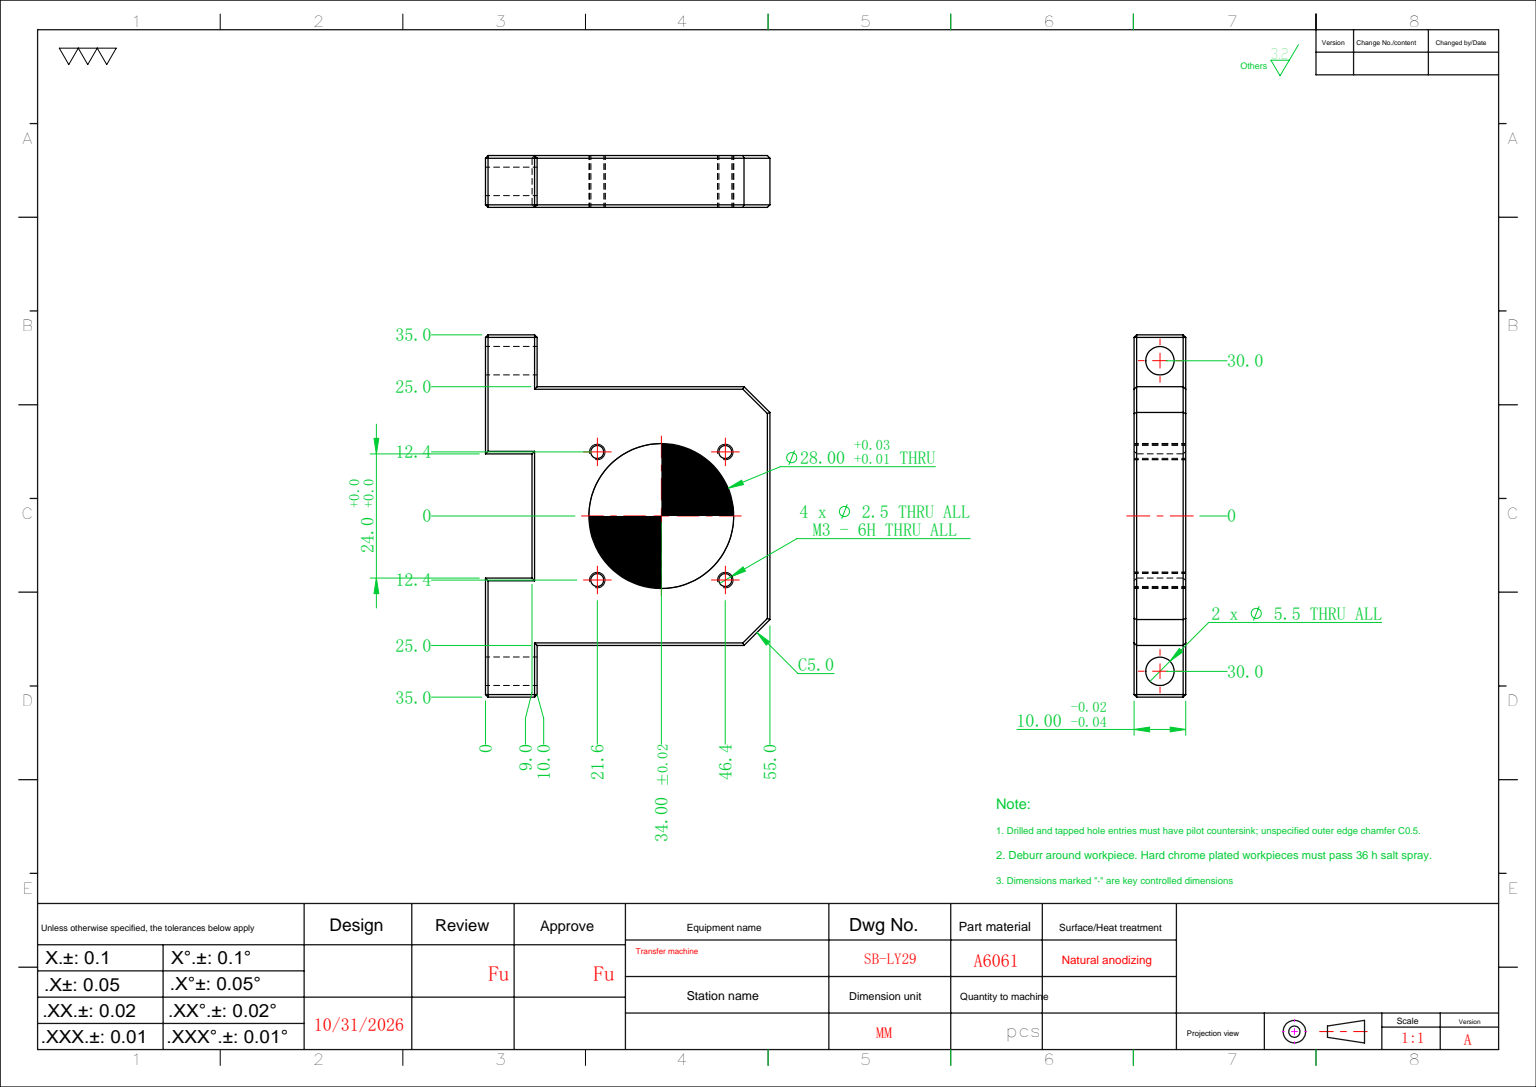
SolidWorks part; units mm, degrees
ref_plane "前视基准面" through (0, 0, 0) normal (0, 0, 1) x (1, 0, 0)
ref_plane "上视基准面" through (0, 0, 0) normal (0, 1, 0) x (1, 0, 0)
ref_plane "右视基准面" through (0, 0, 0) normal (1, 0, 0) x (0, 0, -1)
sketch "草图1" plane through (0, 0, 0) normal (0, 0, 1) x (1, 0, 0)
  line L1 (-35, -27.5) -> (35, -27.5)
  line L2 (-35, -27.5) -> (-35, 27.5)
  line L3 (-35, 27.5) -> (35, 27.5)
  line L4 (35, -27.5) -> (35, 27.5)
  line L5 (-35, -27.5) -> (35, 27.5) construction
  line L6 (-35, 27.5) -> (35, -27.5) construction
  point P0 (0, 0)
  dimension "D1" = 70
  dimension "D2" = 55
extrude "凸台-拉伸1" add sketch "草图1" along normal blind 10
sketch "草图2" plane through (0, 0, 10) normal (0, 0, 1) x (1, 0, 0)
  line L0 (0, 0) -> (0, -35.8295) construction
  line L1 (-35, -27.5) -> (-25, -27.5)
  line L2 (-35, -27.5) -> (-35, 17.5)
  line L3 (-35, 17.5) -> (-25, 17.5)
  line L4 (-25, -27.5) -> (-25, 17.5)
  line L5 (25, -27.5) -> (25, 17.5)
  line L6 (35, 17.5) -> (25, 17.5)
  line L7 (35, -27.5) -> (35, 17.5)
  line L8 (35, -27.5) -> (25, -27.5)
  line L9 (35, 27.5) -> (-35, 27.5) construction
  dimension "D1" = 10
  dimension "D2" = 10
extrude "切除-拉伸1" cut sketch "草图2" against normal through all
sketch "草图3" plane through (0, 0, 0) normal (0, 0, -1) x (-1, 0, 0)
  line L0 (0, 0) -> (0, -40.7468) construction
  line L1 (-35, 27.5) -> (35, 27.5) construction
  circle A0 centre (0, -6.5) radius 14
  dimension "D1" = 28
  dimension "D2" = 34
extrude "切除-拉伸2" cut sketch "草图3" against normal through all
hole_wizard "M3 螺纹孔1" positions "草图8" profile "草图9" tap size "M3" standard "ISO" end condition through all
sketch "草图8" plane through (0, 0, 10) normal (0, 0, 1) x (1, 0, 0)
  line L0 (0, -6.5) -> (0, -34.3856) construction
  line L3 (0, -6.5) -> (-29.4307, -6.5) construction
  point P0 (12.375, -18.875)
  point P2 (-12.375, -18.875)
  point P4 (-12.375, 5.875)
  point P6 (12.375, 5.875)
  dimension "D1" = 24.75
  dimension "D2" = 24.75
sketch "草图9" plane through (12.375, -18.875, 10) normal (1, 0, 0) x (0, -1, 0)
  line L0 (0, 0) -> (0, 10)
  line L1 (0, 10) -> (1.25, 10)
  line L2 (1.25, 10) -> (1.25, 0)
  line L5 (1.25, 0) -> (0, 0)
  line L11 (0, -6.35) -> (0, 107.95) construction
  dimension "通孔螺纹孔钻头直径" = 2.5
  dimension "通孔螺纹孔钻头深度" = 10
cosmetic thread "孔螺蚊线5" parameters "D2"=3
cosmetic thread "孔螺蚊线6" parameters "D2"=3
cosmetic thread "孔螺蚊线7" parameters "D2"=3
cosmetic thread "孔螺蚊线8" parameters "D2"=3
hole_wizard "Ø5.5 (5.5) 直径孔1" positions "草图10" profile "草图11" hole size "Ø5.5" standard "ISO" end condition through all
sketch "草图10" plane through (0, 17.5, 0) normal (0, -1, 0) x (-1, 0, 0)
  line L0 (35, -5) -> (-35, -5) construction
  line L1 (35, 0) -> (35, -10) construction
  line L2 (-35, 0) -> (-35, -10) construction
  line L4 (0, 0) -> (0, -15.7163) construction
  line L5 (-30, 0) -> (-30, -10) construction
  line L6 (-35, 0) -> (-25, 0) construction
  line L7 (-35, -10) -> (-25, -10) construction
  point P0 (-30, -5)
  point P2 (30, -5)
sketch "草图11" plane through (30, 17.5, 5) normal (1, 0, 0) x (0, 0, -1)
  line L0 (0, 0) -> (0, 10)
  line L1 (0, 10) -> (2.75, 10)
  line L2 (2.75, 10) -> (2.75, 0)
  line L5 (2.75, 0) -> (0, 0)
  line L11 (0, -6.35) -> (0, 107.95) construction
  dimension "通孔孔直径" = 5.5
  dimension "通孔孔深度" = 10
chamfer "倒角1" distance 5 angle 45 2 edges at (-25, -27.5, 5) (25, -27.5, 5)
sketch "草图12" plane through (0, 0, 10) normal (0, 0, 1) x (1, 0, 0)
  line L0 (35, 27.5) -> (-35, 27.5) construction
  line L1 (-12, 27.5) -> (12, 27.5)
  line L2 (-12, 27.5) -> (-12, 18.5)
  line L3 (-12, 18.5) -> (12, 18.5)
  line L4 (12, 27.5) -> (12, 18.5)
  line L5 (0, 0) -> (0, 36.1087) construction
  dimension "D1" = 24
  dimension "D2" = 9
extrude "切除-拉伸3" cut sketch "草图12" against normal through all
chamfer "倒角2" distance 0.5 angle 45 32 edges at (-23.5, 27.5, 0) (-30, 17.5, 0) (-25, -2.5, 0) (-22.5, -25, 0) (0, -27.5, 0) (22.5, -25, 0) (25, -2.5, 0) (30, 17.5, 0) (-12, 23, 0) (0, 18.5, 0) (12, 23, 0) (23.5, 27.5, 0) (12, 23, 10) (23.5, 27.5, 10) (0, 18.5, 10) (-12, 23, 10) (-23.5, 27.5, 10) (-35, 27.5, 5) (-35, 22.5, 10) (-35, 22.5, 0) (-35, 17.5, 5) (-30, 17.5, 10) (-25, -2.5, 10) (-22.5, -25, 10) (0, -27.5, 10) (22.5, -25, 10) (25, -2.5, 10) (30, 17.5, 10) (35, 27.5, 5) (35, 22.5, 0) (35, 17.5, 5) (35, 22.5, 10)
